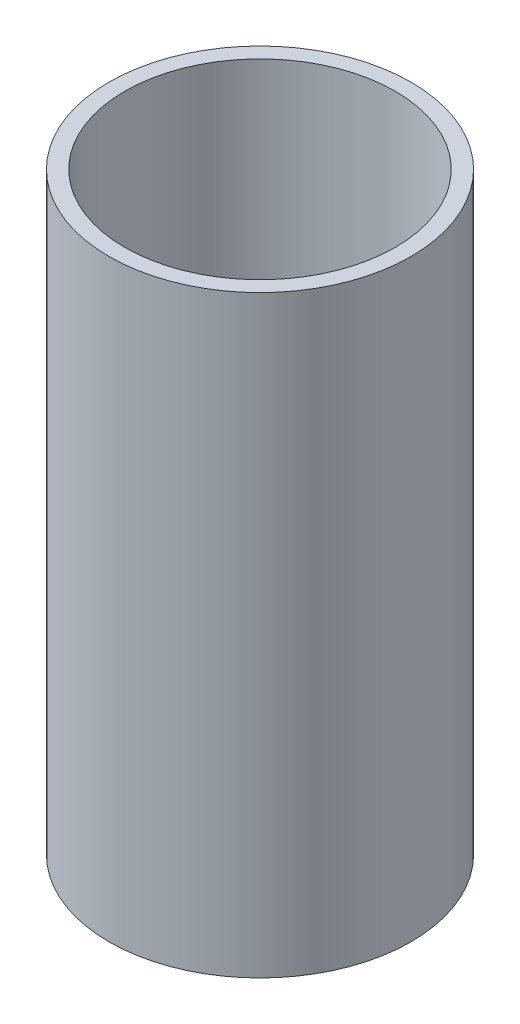
from build123d import *

# Parameters (mm, degrees)
SKETCH1_R           = 11.5
BOSS_EXTRUDE1_DEPTH = 45.2
SKETCH4_R           = 10.3
CUT_EXTRUDE1_DEPTH  = 44
SKETCH5_R           = 9.8
CUT_EXTRUDE2_DEPTH  = 0.9


with BuildPart() as part:
    # Sketch1 → Boss-Extrude1 (new body)
    with BuildSketch(Plane(origin=(0, 0, 0), x_dir=(1, 0, 0), z_dir=(0, 1, 0))):
        with Locations(Location((0, 0, 0), (0, 0, 270))):
            Circle(SKETCH1_R)
    extrude(amount=BOSS_EXTRUDE1_DEPTH)

    # Sketch4 → Cut-Extrude1 (cut)
    with BuildSketch(Plane(origin=(0, 45.2, 0), x_dir=(1, 0, 0), z_dir=(0, 1, 0))):
        with Locations(Location((0, 0, 0), (0, 0, 270))):
            Circle(SKETCH4_R)
    extrude(amount=-CUT_EXTRUDE1_DEPTH, mode=Mode.SUBTRACT)

    # Sketch5 → Cut-Extrude2 (cut)
    with BuildSketch(Plane.XZ):
        with Locations(Location((0, 0, 0), (0, 0, 270))):
            Circle(SKETCH5_R)
    extrude(amount=-CUT_EXTRUDE2_DEPTH, mode=Mode.SUBTRACT)


solid = part.part
